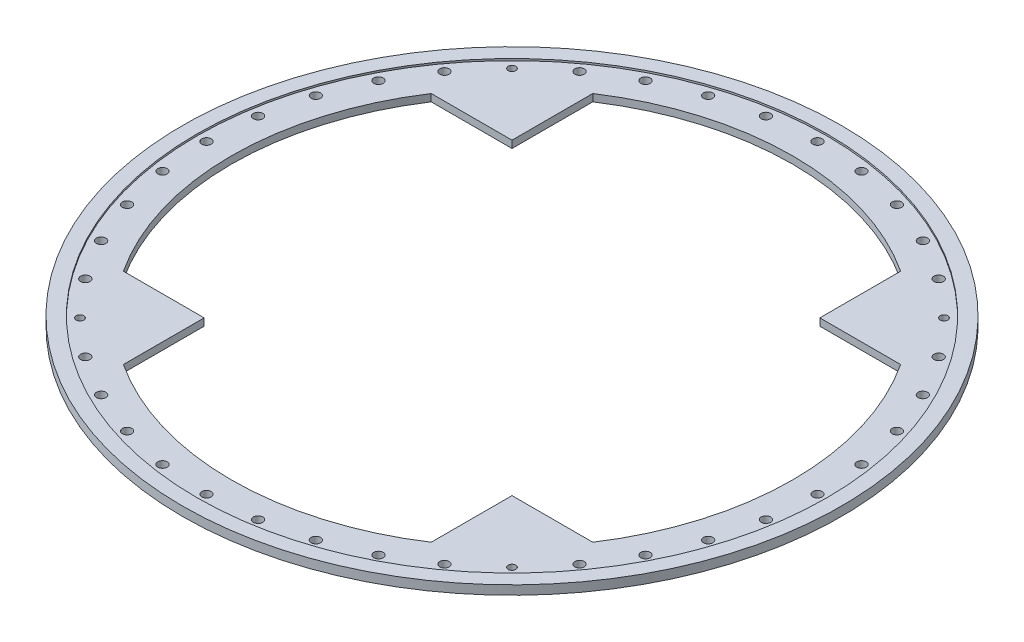
SolidWorks part; units mm, degrees
material "XRAAT"
ref_plane "前视基准面" through (0, 0, 0) normal (0, 0, 1) x (1, 0, 0)
ref_plane "上视基准面" through (0, 0, 0) normal (0, 1, 0) x (1, 0, 0)
ref_plane "右视基准面" through (0, 0, 0) normal (1, 0, 0) x (0, 0, -1)
sketch "草图1" plane through (0, 0, 0) normal (0, 1, 0) x (1, 0, 0)
  line L0 (-425, 425) -> (-425, 648.0741)
  line L1 (425, -425) -> (-425, -425)
  line L2 (425, -425) -> (425, 425)
  line L3 (425, 425) -> (-425, 425)
  line L4 (-425, -425) -> (-425, 425)
  line L5 (425, -425) -> (-425, 425) construction
  line L6 (425, 425) -> (-425, -425) construction
  line L7 (-425, 425) -> (-648.0741, 425)
  line L8 (-425, 0) -> (0, 0) construction
  line L9 (0, 0) -> (0, 425) construction
  line L10 (-425, -425) -> (-425, -648.0741)
  line L11 (-425, -425) -> (-648.0741, -425)
  line L12 (425, -425) -> (425, -648.0741)
  line L13 (425, -425) -> (648.0741, -425)
  line L14 (425, 425) -> (648.0741, 425)
  line L15 (425, 425) -> (425, 648.0741)
  line L16 (489, 611) -> (611, 489) construction
  line L17 (-489, 489) -> (-611, 489)
  line L18 (-489, 489) -> (-489, 611)
  line L19 (-489, 611) -> (-611, 611)
  line L20 (-611, 489) -> (-611, 611)
  line L21 (-489, 489) -> (-611, 611) construction
  line L22 (-489, 611) -> (-611, 489) construction
  line L23 (489, 489) -> (611, 611) construction
  line L24 (611, 489) -> (611, 611)
  line L25 (489, 611) -> (611, 611)
  line L26 (489, 489) -> (489, 611)
  line L27 (489, 489) -> (611, 489)
  line L28 (489, -489) -> (611, -611) construction
  line L29 (489, -611) -> (611, -489) construction
  line L30 (489, -489) -> (611, -489)
  line L31 (489, -489) -> (489, -611)
  line L32 (489, -611) -> (611, -611)
  line L33 (611, -489) -> (611, -611)
  line L34 (-489, -611) -> (-611, -489) construction
  line L35 (-489, -489) -> (-611, -611) construction
  line L36 (-611, -489) -> (-611, -611)
  line L37 (-489, -611) -> (-611, -611)
  line L38 (-489, -489) -> (-489, -611)
  line L39 (-489, -489) -> (-611, -489)
  circle A0 centre (0, 0) radius 910
  circle A1 centre (0, 0) radius 775
  point P18 (-550, 550)
  point P28 (550, 550)
  point P33 (550, -550)
  point P38 (-550, -550)
  dimension "D1" = 1820
  dimension "D2" = 1550
  dimension "D3" = 850
  dimension "D4" = 122
  dimension "D5" = 1100
  dimension "D6" = 1100
extrude "凸台-拉伸1" add sketch "草图1" along normal blind 25 contours A0 A1 L30 L33 L32 L31 L38 L37 L36 L39 L17 L20 L19 L18 L26 L25 L24 L27 | L30 A1 L13 L12 L31 | L11 A1 L39 L38 L10 | L0 A1 L18 L17 L7 | L14 A1 L27 L26 L15 | L18 A1 L17 | A1 L18 L19 L20 L17 | L27 A1 L26 | A1 L27 L24 L25 L26 | A1 L31 L32 L33 L30 | L31 A1 L30 | A1 L39 L36 L37 L38 | L39 A1 L38
sketch "草图2" plane through (0, 25, 0) normal (0, 1, 0) x (1, 0, 0)
  circle A0 centre (0, 0) radius 870
  dimension "D1" = 1740
extrude "切除-拉伸1" cut sketch "草图2" against normal blind 5
hole_wizard "Ø26 直径孔1" positions "草图3" profile "草图4" hole size "Ø12.0" standard "GB" end condition up to next
sketch "草图3" plane through (0, 20, 0) normal (0, 1, 0) x (1, 0, 0)
  line L0 (0, 0) -> (0, 843.5) construction
  circle A0 centre (0, 0) radius 843.5 construction
  point P0 (0, 843.5)
  dimension "D1" = 1687
sketch "草图4" plane through (0, 20, -843.5) normal (1, 0, 0) x (0, 0, 1)
  line L0 (0, 0) -> (0, 20)
  line L1 (0, 20) -> (13, 20)
  line L2 (13, 20) -> (13, 0)
  line L5 (13, 0) -> (0, 0)
  line L11 (0, -6.35) -> (0, 107.95) construction
  dimension "通孔孔直径" = 26
  dimension "通孔孔深度" = 20
pattern_circular "阵列(圆周)1" count 40 over 360 about axis through (0, 0, 0) along (0, 1, 0) skipping 5, 15, 25, 35 of "Ø26 直径孔1"
hole_wizard "M24 螺纹孔1" positions "草图5" profile "草图6" tap size "M24" standard "GB" end condition up to next
sketch "草图5" plane through (0, 20, 0) normal (0, 1, 0) x (1, 0, 0)
  line L0 (-596.4446, 596.4446) -> (0, 0) construction
  circle A0 centre (0, 0) radius 843.5 construction
  point P0 (-596.4446, 596.4446)
  point P16 (596.4446, 596.4446)
  point P17 (596.4446, -596.4446)
  point P18 (-596.4446, -596.4446)
  dimension "D1" = 45
  dimension "D2" = 4
sketch "草图6" plane through (-596.4446, 20, -596.4446) normal (1, 0, 0) x (0, 0, 1)
  line L0 (0, 0) -> (0, 20)
  line L1 (0, 20) -> (10.5, 20)
  line L2 (10.5, 20) -> (10.5, 0)
  line L5 (10.5, 0) -> (0, 0)
  line L11 (0, -6.35) -> (0, 107.95) construction
  dimension "通孔螺纹孔钻头直径" = 21
  dimension "通孔螺纹孔钻头深度" = 20
cosmetic thread "孔螺蚊线1" parameters "D2"=24
cosmetic thread "孔螺蚊线2" parameters "D2"=24
cosmetic thread "孔螺蚊线3" parameters "D2"=24
cosmetic thread "孔螺蚊线4" parameters "D2"=24
